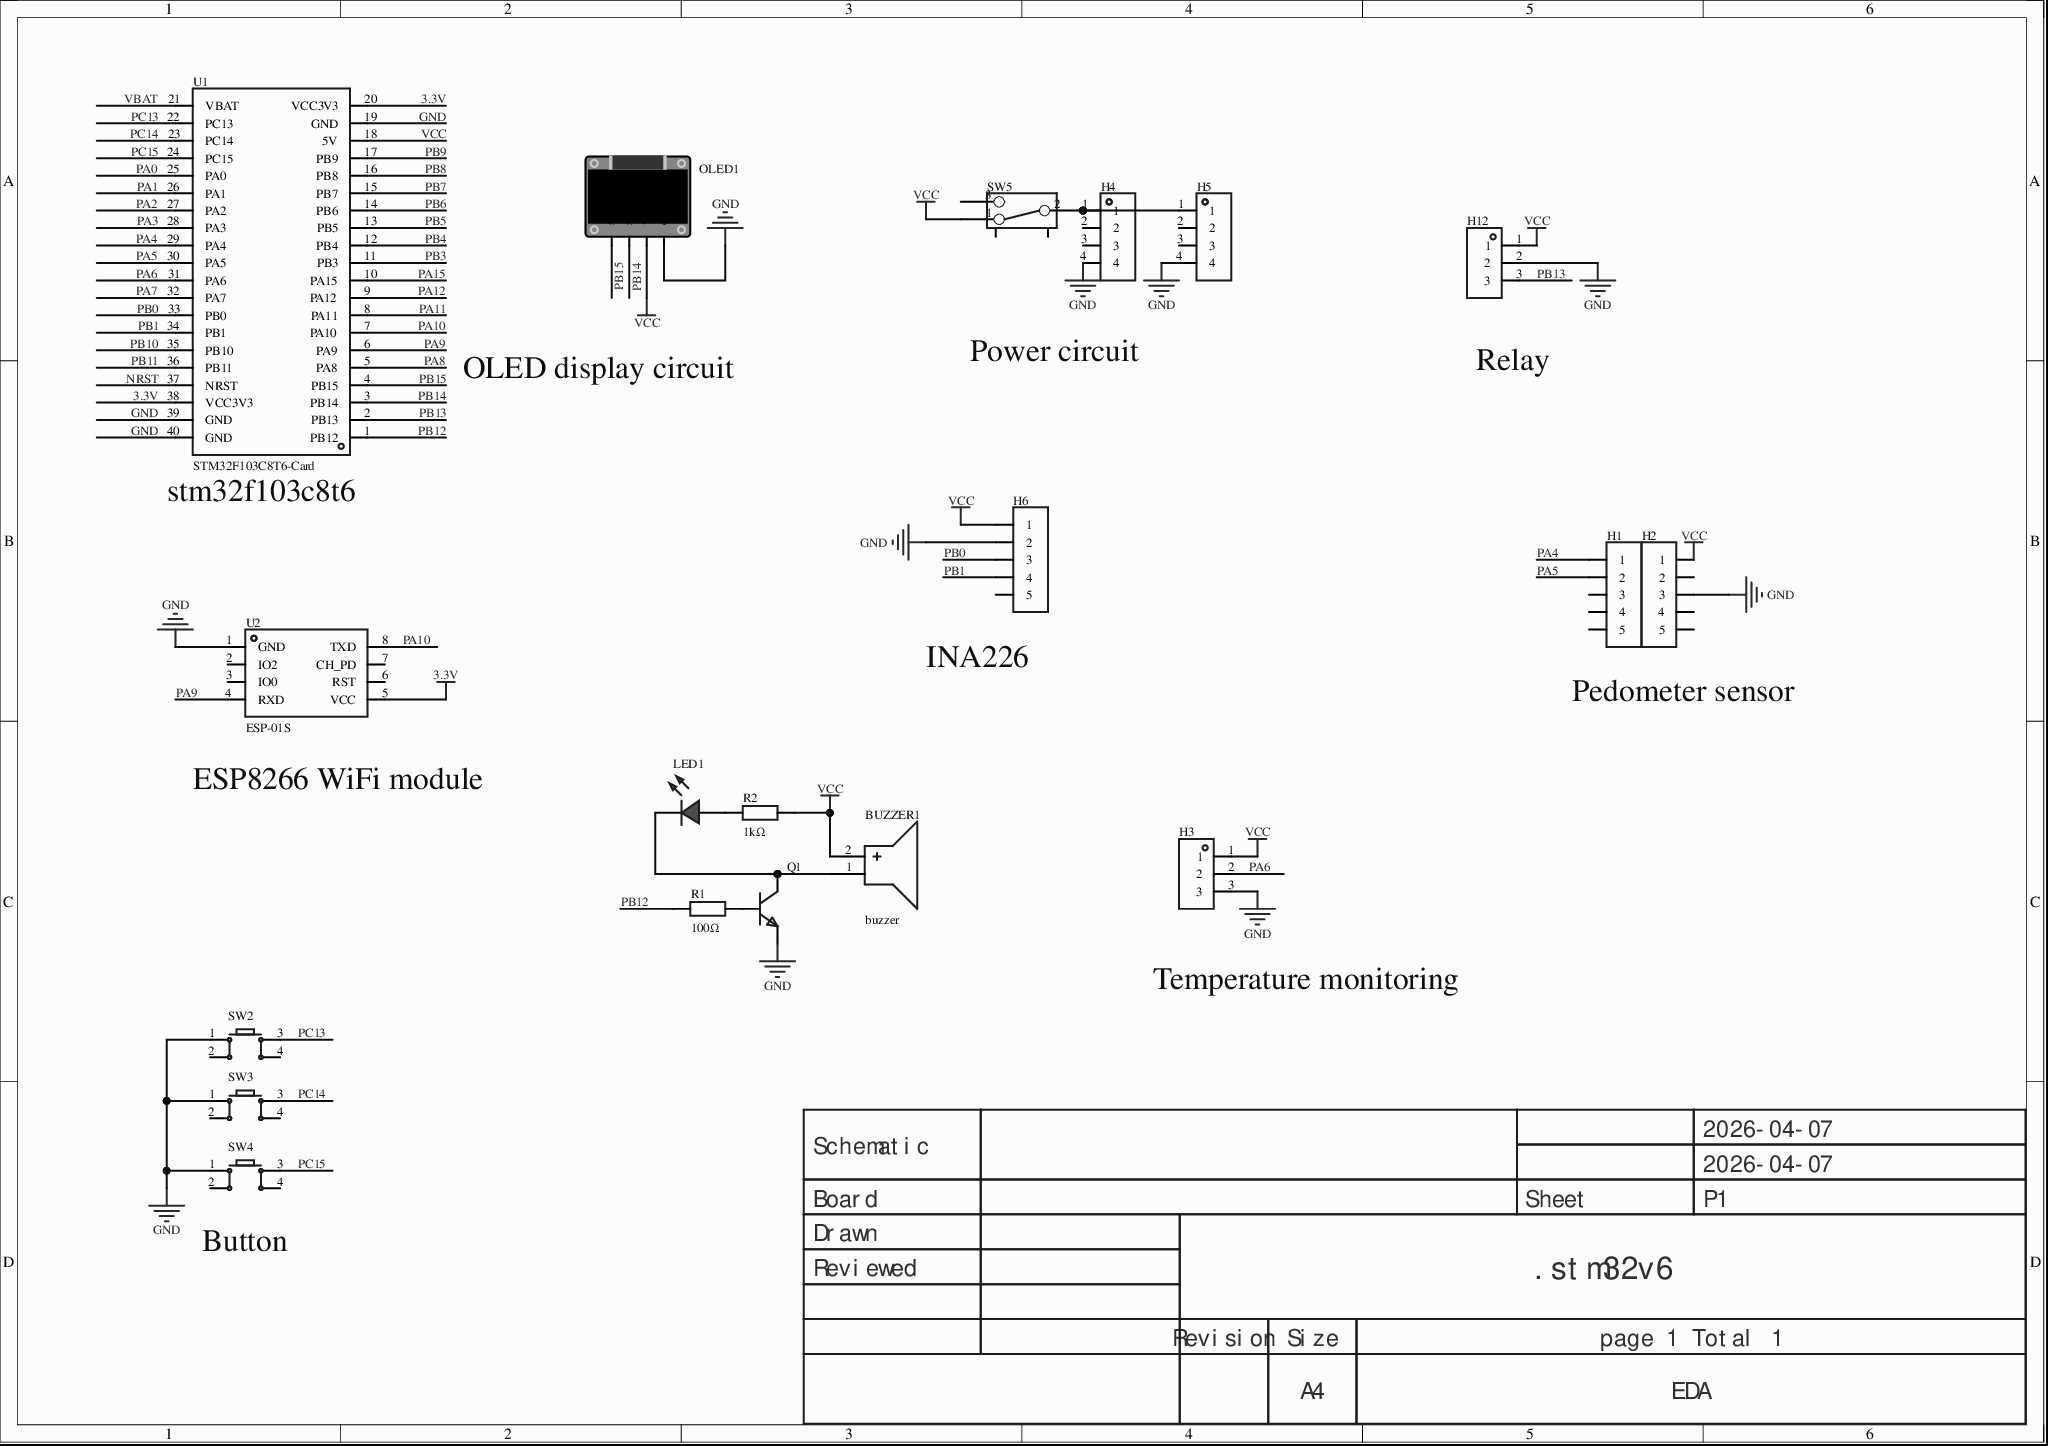
[diagram p0: MISC89063-3.schdoc]
# Altium project MISC89063-2.PrjPcb
1 sheet, 19 parts. Net scope: global (net labels, ports and power ports of the same name join across sheets).
Board file: MISC89063.pcbdoc

## Sheet MISC89063-3.schdoc
size 297 x 209 mm; Version: V1.0; @Project Name: MISC89063; @Page Count: 1; @Update Date: 2026-04-07; @Create Date: 2026-04-07; @Schematic Name: MISC89063; @Page No: 1; @Create Time: 23:22:16; @Update Time: 17:32:40; @Board Name: MISC89063

### Parts
BUZZER1  buzzer  [BUZ-TH_BD12.0-P6.00-D0.9-RD]
H1  (no value)  [HDR-TH_5P-P2.54-V-F]
H2  (no value)  [HDR-TH_5P-P2.54-V-F]
H3  (no value)  [HDR-TH_3P-P2.54-V-F]
H4  (no value)  [HDR-TH_4P-P2.54-V-F]
H5  (no value)  [HDR-TH_4P-P2.54-V-F]
H6  (no value)  [HDR-TH_5P-P2.54-V-F]
H12  (no value)  [HDR-TH_3P-P2.54-V-F]
LED1  (no value)  [LED_TH-3mm]
OLED1  (no value)  [0.96OLED_4P]
Q1  (no value)  [S8050_TO_92]
R1  100Ω  [Res_1/8W]
R2  1kΩ  [Res_1/8W]
SW2  (no value)  [SW-TH_4P-L6.0-W6.0-P4.50-LS6.5]
SW3  (no value)  [SW-TH_4P-L6.0-W6.0-P4.50-LS6.5]
SW4  (no value)  [SW-TH_4P-L6.0-W6.0-P4.50-LS6.5]
SW5  (no value)  [拨动开关]
U1  STM32F103C8T6-Card  [CONN-TH_L53.3-W22.9_STM32F103C8T6-CARD]
U2  ESP-01S  [WIFIM-TH_ESP-01S]

### Nets
3.3V: U1.20(VCC3V3) U1.38(VCC3V3) U2.5(VCC)
GND: H2.3 H3.3 H4.4 H5.4 H6.2 H12.2 OLED1.1(GND) Q1.1(E) SW2.1 SW3.1 SW4.1 U1.19(GND) U1.39(GND) U1.40(GND) U2.1(GND)
VCC: BUZZER1.2(+) H2.1 H3.1 H6.1 H12.1 OLED1.2(VCC) R2.2 SW5.1 U1.18(5V)
NRST: U1.37(NRST)
PA0: U1.25(PA0)
PA1: U1.26(PA1)
PA2: U1.27(PA2)
PA3: U1.28(PA3)
PA4: H1.1 U1.29(PA4)
PA5: H1.2 U1.30(PA5)
PA6: H3.2 U1.31(PA6)
PA7: U1.32(PA7)
PA8: U1.5(PA8)
PA9: U1.6(PA9) U2.4(RXD)
PA10: U1.7(PA10) U2.8(TXD)
PA11: U1.8(PA11)
PA12: U1.9(PA12)
PA15: U1.10(PA15)
PB0: H6.3 U1.33(PB0)
PB1: H6.4 U1.34(PB1)
PB3: U1.11(PB3)
PB4: U1.12(PB4)
PB5: U1.13(PB5)
PB6: U1.14(PB6)
PB7: U1.15(PB7)
PB8: U1.16(PB8)
PB9: U1.17(PB9)
PB10: U1.35(PB10)
PB11: U1.36(PB11)
PB12: R1.1 U1.1(PB12)
PB13: H12.3 U1.2(PB13)
PB14: OLED1.3(SCL) U1.3(PB14)
PB15: OLED1.4(SDA) U1.4(PB15)
PC13: SW2.3 U1.22(PC13)
PC14: SW3.3 U1.23(PC14)
PC15: SW4.3 U1.24(PC15)
VBAT: U1.21(VBAT)
NetBUZZER1_1: BUZZER1.1(-) LED1.2(A) Q1.3(C)
NetH4_1: H4.1 H5.1 SW5.2
NetLED1_1: LED1.1(C) R2.1
NetQ1_2: Q1.2(B) R1.2

Not connected (* = marked no-connect by the designer): H1 3 4 5; H2 2 4 5; H4 2 3; H5 2 3; H6 5; SW2 2 4; SW3 2 4; SW4 2 4; SW5 3 4 5; U2 2(IO2)* 3(IO0)* 6(RST)* 7(CH_PD)*

### Notes on the sheet
- OLED display circuit
- Power circuit
- (near H12) Relay
- (near U1) stm32f103c8t6
- (near H6) INA226
- Pedometer sensor
- (near U2) ESP8266 WiFi module
- Temperature monitoring
- (near SW4) Button
- 2026-04-07
- Schematic
- Board
- Sheet
- P1
- Drawn
- Reviewed
- .stm32v6
- Revision
- Size
- A4
- page 1 Total 1
- EDA

### Library data of the parts
BUZZER1 = buzzer: AddInBom: yes; ModelId: af17e4151ed84fc2a628230bf23763630819f05c4eef4c71ace90d822a990e87; ModelTransform: 472.44,472.176,0,270,0,0,0,0,-196.85; Symbol: BUZZER; Device: buzzer; LCSC Part Name: buzzer; SupplierPart: C9900014030; ManufacturerPart: buzzer; Supplier Footprint: buzzer; JLCPCB Part Class: Extended Part; Supplier: LCSC; ConvertToPcb: yes; FootprintName: BUZ-TH_BD12.0-P6.00-D0.9-RD; ModelName: BUZ-TH_BD12.0-P6.00-D0.9-RD
H1 H2 H6 = HDR-F_2.54_1x5P: Symbol: Header-Female-2.54_1x5; ConvertToPcb: yes; ModelId: f49cb6116a3d45e5a64915bf3e00773f; ModelTransform: 519.684,98.464,0,0,0,0,0,0,-124.016; Device: HDR-F_2.54_1x5P; AddInBom: yes; SupplierPart: C50950; Supplier Footprint: 插件; FootprintName: HDR-TH_5P-P2.54-V-F; ModelName: HDR-TH_5P-P2.54-V-F
H3 H12 = HDR-F_2.54_1x3P: Symbol: PM254V-11-03-H85; 3D Model: f3b3cc5aae9641bf9e56fc160cef875b; 3D Model Transform: 299.9994,100,0,0,0,0,0,0,-118.11; ConvertToPcb: yes; ModelName: HDR2.54-F-LI-1X3P; Device: HDR-F_2.54_1x3P; Supplier Part: C541850; Supplier Footprint: 插件; AddInBom: yes; FootprintName: HDR-TH_3P-P2.54-V-F
H4 H5 = HDR-F_2.54_1x4P: Symbol: 2.54-1*4P female; ConvertToPcb: yes; ModelId: d187812051054f85879fcaa51a310d8e0819f05c4eef4c71ace90d822a990e87; ModelTransform: 419.6842,98.464,0,0,0,0,0,0,-118.11; Device: HDR-F_2.54_1x4P; AddInBom: yes; SupplierPart: C2718488; Supplier Footprint: 插件; FootprintName: HDR-TH_4P-P2.54-V-F; ModelName: HDR-TH_4P-P2.54-V-F
LED1 = LED_TH-R_3mm: ConvertToPcb: yes; ModelId: a497c992633541038a38947cdc58012f0819f05c4eef4c71ace90d822a990e87; ModelName: LED-TH-3mm_R; ModelTransform: 141.274,153.327,0,0,0,0,-5.984,0,-137.795; Symbol: LED_TH-R; Device: LED_TH-R_3mm; AddInBom: yes; FootprintName: LED_TH-3mm; Supplier Footprint: 插件
OLED1 = 0.96OLED模块_4P: Symbol: 0.96OLED module_4P; ConvertToPcb: yes; ModelId: 79c000fdb68d45a296c2e9bedf4f9055; ModelTransform: 1393.69792,1318.895,0,0,0,0,0,-560.079,-137.795; Device: 0.96OLED module_4P; AddInBom: yes; FootprintName: 0.96OLED_4P; Supplier Footprint: 插件; ModelName: 0.96OLED_4P
Q1 = S8050_TO_NPN: ConvertToPcb: yes; ModelId: aafe8e06f2154e7c93506efd0d6632dd; ModelName: TO-92-3_L4.9-W3.7-P1.27-L; ModelTransform: 180.78,141.44,417.3,0,0,0,0,0,-200; Symbol: S8050_TO_NPN; Device: S8050_TO_NPN; AddInBom: yes; Supplier Footprint: TO-92; FootprintName: S8050_TO_92
R1 R2 = Res_AXIAL-1/8W: Symbol: Resistor; ConvertToPcb: yes; ModelId: b2b5ae7ae4c642178fe0039925c86a3f0819f05c4eef4c71ace90d822a990e87; ModelName: RES-TH_BD1.8-L3.2-P7.20-D0.4; ModelTransform: 282.86,66.88,253.09,0,0,0,0,0,-191; Device: Res_AXIAL-1/8W; AddInBom: yes; Supplier Footprint: 轴向引线; FootprintName: Res_1/8W
  R1: Value: 100Ω
  R2: Value: 1kΩ
SW2-SW4 = Key_TH_6x6x6: 触点电流:50mA;额定电压(DC):12V;绝缘电阻:100MΩ;电路结构:单刀单掷;安装方式:直插;按钮形状:圆形按钮;按钮/盖帽颜色:黑色;作用力:260gf@±30gf;工作温度:-25℃~+70℃;引脚样式:PC引脚;开关长度:6mm;开关宽度:6mm;开关高度:6mm;带支架:否;; Symbol: Tact switch; AddInBom: yes; ModelId: 20eee248bc684ccd8cbdbb1d0d91ec6f0819f05c4eef4c71ace90d822a990e87; ModelName: SW-TH_4P-L6.0-W6.0-H5.0-LS6.5-P4.50; ModelTransform: 236.22,323.03,0,90,0,0,0,0,-137.795; Device: Key_TH_6x6x6; ConvertToPcb: yes; FootprintName: SW-TH_4P-L6.0-W6.0-P4.50-LS6.5; Supplier Footprint: 插件
SW5 = 拨动开关_正: Symbol: Toggle switch; Device: Toggle switch_positive; ConvertToPcb: yes; ModelId: 4321fe59a4074cbfb4989553f297c68f0819f05c4eef4c71ace90d822a990e87; ModelName: SW-TH_SS-12D02-VG4; ModelTransform: 370.09,208.7,472.35,0,0,0,0,0,-110; AddInBom: yes; Supplier Footprint: 插件; FootprintName: Toggle switch
U1 = STM32F103C8T6-Card: AddInBom: yes; Symbol: STM32F103C8T6-CARD; Device: STM32F103C8T6-Card; LCSC Part Name: STM32F103C8T6-Card; SupplierPart: C9900077949; ManufacturerPart: STM32F103C8T6-Card; Supplier Footprint: 插件; Supplier: LCSC; ConvertToPcb: yes; FootprintName: CONN-TH_L53.3-W22.9_STM32F103C8T6-CARD
U2 = ESP-01S_C111009: 3D Model: eb7175da78ae48b3b1568cfe3027405f0819f05c4eef4c71ace90d822a990e87; 3D Model Transform: 582.676,976.37608,0,0,0,0,0,388.346,-118.11; AddInBom: yes; Symbol: ESP-01S; Device: ESP-01S_C111009; LCSC Part Name: ESP-01S; Supplier Part: C111009; Manufacturer Part: ESP-01S; Supplier Footprint: -; JLCPCB Part Class: Extended Part; Supplier: LCSC; ConvertToPcb: yes; FootprintName: WIFIM-TH_ESP-01S; ModelName: WIFIM-TH_ESP-01S